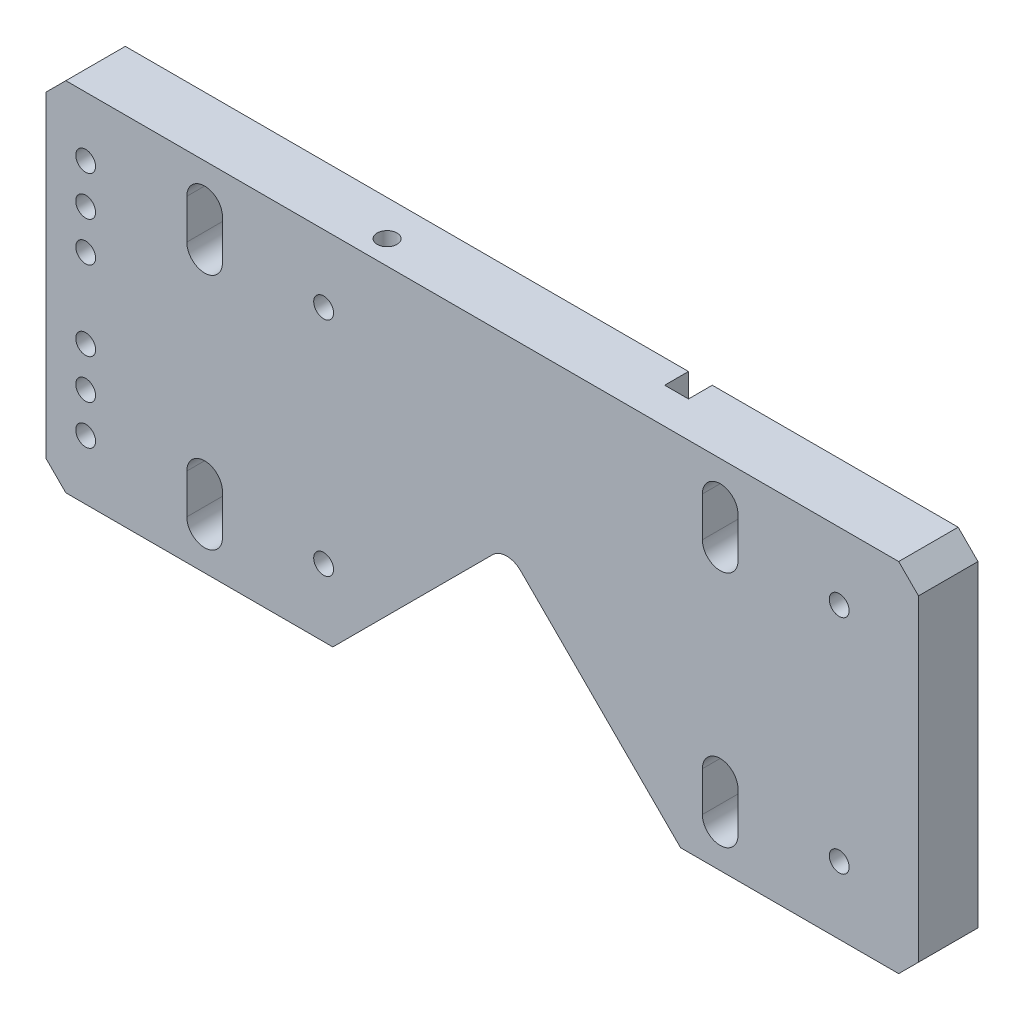
SolidWorks part; units mm, degrees
material "45"
ref_plane "Front Plane" through (0, 0, 0) normal (0, 0, 1) x (1, 0, 0)
ref_plane "Top Plane" through (0, 0, 0) normal (0, 1, 0) x (1, 0, 0)
ref_plane "Right Plane" through (0, 0, 0) normal (1, 0, 0) x (0, 0, -1)
sketch "Sketch1" plane through (0, 0, 0) normal (0, 0, 1) x (1, 0, 0)
  line L1 (0, 0) -> (220, 0)
  line L2 (0, 0) -> (0, 90)
  line L3 (0, 90) -> (220, 90)
  line L4 (220, 0) -> (220, 90)
  dimension "D1" = 90
  dimension "D2" = 220
extrude "Boss-Extrude1" add sketch "Sketch1" along normal blind 15
hole_wizard "M6 Tapped Hole1" positions "Sketch3" profile "Sketch2" tap size "M6" standard "Gb"
sketch "Sketch3" plane through (0, 0, 15) normal (0, 0, 1) x (1, 0, 0)
  line L0 (135, 90) -> (135, 45) construction
  line L2 (135, 45) -> (220, 45) construction
  line L3 (220, 0) -> (220, 90) construction
  line L5 (220, 90) -> (0, 90) construction
  point P0 (70, 73)
  point P2 (70, 17)
  point P4 (200, 73)
  point P6 (200, 17)
  dimension "D1" = 56
  dimension "D2" = 130
  dimension "D3" = 20
sketch "Sketch2" plane through (70, 73, 15) normal (1, 0, 0) x (0, -1, 0)
  line L0 (0, 0) -> (0, 16.5022)
  line L1 (0, 16.5022) -> (2.5, 15)
  line L2 (2.5, 15) -> (2.5, 0)
  line L5 (2.5, 0) -> (0, 0)
  line L10 (0, 16.5022) -> (-2.5, 15) construction
  line L11 (0, -6.35) -> (0, 107.95) construction
  dimension "螺纹孔钻头直径" = 5
  dimension "螺纹孔钻头深度" = 15
  dimension "导头角度" = 118
cosmetic thread "Hole thread 1" parameters "D1"=12, "D2"=6
cosmetic thread "Hole thread 2" parameters "D1"=12, "D2"=6
cosmetic thread "Hole thread 3" parameters "D1"=12, "D2"=6
cosmetic thread "Hole thread 4" parameters "D1"=12, "D2"=6
sketch "Sketch4" plane through (0, 0, 15) normal (0, 0, 1) x (1, 0, 0)
  line L0 (40, 80) -> (40, 70) construction
  line L1 (44.5, 80) -> (44.5, 70)
  line L2 (35.5, 80) -> (35.5, 70)
  line L3 (40, 20) -> (40, 10) construction
  line L4 (44.5, 20) -> (44.5, 10)
  line L5 (35.5, 20) -> (35.5, 10)
  line L6 (170, 80) -> (170, 70) construction
  line L7 (174.5, 80) -> (174.5, 70)
  line L8 (165.5, 80) -> (165.5, 70)
  line L9 (170, 20) -> (170, 10) construction
  line L10 (174.5, 20) -> (174.5, 10)
  line L11 (165.5, 20) -> (165.5, 10)
  line L12 (0, 45) -> (80, 45) construction
  line L13 (0, 90) -> (0, 0) construction
  arc A0 (44.5, 80) -> (35.5, 80) centre (40, 80) ccw
  arc A1 (35.5, 70) -> (44.5, 70) centre (40, 70) ccw
  arc A2 (44.5, 20) -> (35.5, 20) centre (40, 20) ccw
  arc A3 (35.5, 10) -> (44.5, 10) centre (40, 10) ccw
  arc A4 (174.5, 80) -> (165.5, 80) centre (170, 80) ccw
  arc A5 (165.5, 70) -> (174.5, 70) centre (170, 70) ccw
  arc A6 (174.5, 20) -> (165.5, 20) centre (170, 20) ccw
  arc A7 (165.5, 10) -> (174.5, 10) centre (170, 10) ccw
  circle A8 centre (200, 73) radius 2.5 construction
  circle A9 centre (70, 73) radius 2.5 construction
  point P2 (40, 75)
  point P7 (40, 15)
  point P14 (170, 75)
  point P21 (170, 15)
  dimension "D1" = 4.5
  dimension "D3" = 30
  dimension "D5" = 30
  dimension "D2" = 10
  dimension "D4" = 60
extrude "Cut-Extrude1" cut sketch "Sketch4" against normal through all
sketch "Sketch5" plane through (0, 0, 15) normal (0, 0, 1) x (1, 0, 0)
  line L0 (72.3188, 0) -> (116.1594, 43.8406)
  line L1 (72.3188, 0) -> (116.1594, -43.8406)
  line L2 (116.1594, 43.8406) -> (160, 0)
  line L3 (116.1594, -43.8406) -> (160, 0)
  line L4 (0, 0) -> (220, 0) construction
  line L6 (0, 0) -> (220, 0) construction
  line L7 (220, 0) -> (220, 90) construction
  dimension "D1" = 60
  dimension "D2" = 62
  dimension "D3" = 45
extrude "Cut-Extrude2" cut sketch "Sketch5" against normal through all
hole_wizard "M6 Tapped Hole2" positions "Sketch7" profile "Sketch6" tap size "M6" standard "Gb"
sketch "Sketch7" plane through (0, 90, 0) normal (0, 1, 0) x (1, 0, 0)
  line L0 (220, -15) -> (0, -15) construction
  line L1 (0, -15) -> (0, 0) construction
  point P0 (80, -9)
  point P5 (0, -7.5)
  dimension "D1" = 6
  dimension "D2" = 80
sketch "Sketch6" plane through (80, 90, 9) normal (1, 0, 0) x (0, 0, 1)
  line L0 (0, 0) -> (0, 16.5022)
  line L1 (0, 16.5022) -> (2.5, 15)
  line L2 (2.5, 15) -> (2.5, 0)
  line L5 (2.5, 0) -> (0, 0)
  line L10 (0, 16.5022) -> (-2.5, 15) construction
  line L11 (0, -6.35) -> (0, 107.95) construction
  dimension "螺纹孔钻头直径" = 5
  dimension "螺纹孔钻头深度" = 15
  dimension "导头角度" = 118
cosmetic thread "Hole thread 5" parameters "D1"=12, "D2"=6
chamfer "Chamfer1" distance 5 angle 45 4 edges at (220, 90, 7.5) (0, 90, 7.5) (220, 0, 7.5) (0, 0, 7.5)
fillet "Fillet1" radius 5 1 edges at (116.1594, 43.8406, 7.5)
sketch "Sketch8" plane through (0, 0, 15) normal (0, 0, 1) x (1, 0, 0)
  line L0 (40, 84.5) -> (40, 65.5) construction
  line L2 (40, 24.5) -> (40, 5.5) construction
  line L4 (170, 84.5) -> (170, 65.5) construction
  line L6 (170, 24.5) -> (170, 5.5) construction
  circle A0 centre (40, 75) radius 4
  circle A1 centre (40, 15) radius 4
  circle A2 centre (170, 15) radius 4
  circle A3 centre (170, 75) radius 4
  arc A4 (44.5, 80) -> (35.5, 80) centre (40, 80) ccw construction
  arc A6 (44.5, 20) -> (35.5, 20) centre (40, 20) ccw construction
  arc A9 (35.5, 10) -> (44.5, 10) centre (40, 10) ccw construction
  arc A10 (165.5, 70) -> (174.5, 70) centre (170, 70) ccw construction
  arc A11 (174.5, 80) -> (165.5, 80) centre (170, 80) ccw construction
  arc A12 (174.5, 20) -> (165.5, 20) centre (170, 20) ccw construction
  arc A13 (165.5, 10) -> (174.5, 10) centre (170, 10) ccw construction
  arc A14 (35.5, 70) -> (44.5, 70) centre (40, 70) ccw construction
  dimension "D1" = 8
sketch "Sketch10" plane through (0, 0, 0) normal (0, 0, -1) x (-1, 0, 0)
  line L0 (-150, 0) -> (-150, 90) construction
  line L1 (-153, 0) -> (-153, 90)
  line L2 (-147, 0) -> (-147, 90)
  line L4 (-220, 5) -> (-220, 85) construction
  line L5 (-215, 90) -> (-5, 90) construction
  line L6 (-160, 0) -> (-215, 0) construction
  arc A0 (-153, 0) -> (-147, 0) centre (-150, 0) ccw
  arc A1 (-147, 90) -> (-153, 90) centre (-150, 90) ccw
  point P2 (-150, 45)
  dimension "D4" = 3
  dimension "D3" = 70
extrude "Cut-Extrude3" cut sketch "Sketch10" against normal blind 6
sketch "Sketch11" plane through (0, 0, 15) normal (0, 0, 1) x (1, 0, 0)
  line L0 (0, 45) -> (26.7349, 45) construction
  line L1 (0, 85) -> (0, 5) construction
  circle A0 centre (10, 55) radius 2.5
  circle A1 centre (10, 35) radius 2.5
  circle A2 centre (10, 25) radius 2.5
  circle A3 centre (10, 65) radius 2.5
  circle A4 centre (10, 75) radius 2.5
  circle A5 centre (10, 15) radius 2.5
  dimension "D1" = 5
  dimension "D2" = 10
  dimension "D3" = 20
  dimension "D4" = 10
  dimension "D5" = 10
extrude "Cut-Extrude4" cut sketch "Sketch11" against normal through all
sketch "Sketch12" plane through (0, 0, 6) normal (0, 0, -1) x (-1, 0, 0)
  line L0 (-150, 90) -> (-150, 75) construction
  line L1 (-147, 90) -> (-153, 90) construction
  line L2 (-150, 75) -> (-150, 25) construction
  circle A0 centre (-150, 75) radius 3
  circle A1 centre (-150, 25) radius 3
  dimension "D3" = 6
  dimension "D1" = 15
  dimension "D2" = 50
